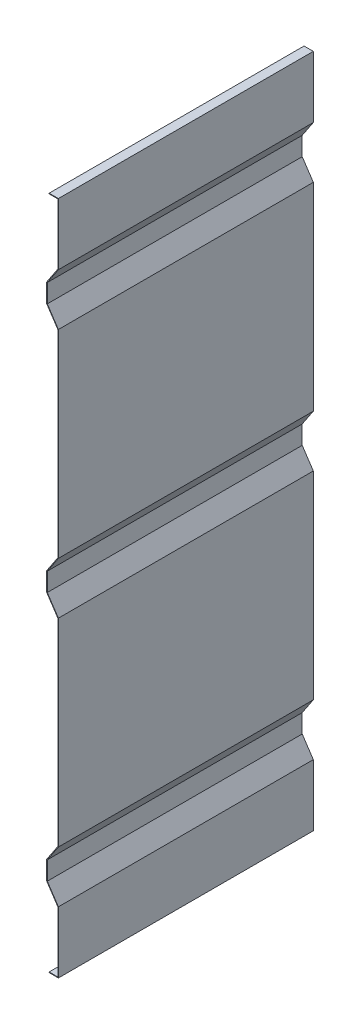
SolidWorks part; units mm, degrees
ref_plane "Front Plane" through (0, 0, 0) normal (0, 0, 1) x (1, 0, 0)
ref_plane "Top Plane" through (0, 0, 0) normal (0, 1, 0) x (1, 0, 0)
ref_plane "Right Plane" through (0, 0, 0) normal (1, 0, 0) x (0, 0, -1)
other "Configuration Table"
sketch "Sketch1" plane through (0, 0, 0) normal (0, 0, 1) x (1, 0, 0)
  line L0 (0, 1095) -> (-30, 1095)
  line L1 (0, 1095) -> (0, 895)
  line L2 (0, 895) -> (-36, 841)
  line L3 (-36, 841) -> (-36, 781)
  line L4 (-36, 781) -> (0, 727)
  line L5 (0, 84) -> (-36, 30)
  line L6 (-36, -30) -> (0, -84)
  line L7 (-36, 30) -> (-36, -30)
  line L8 (-36, 0) -> (85.9436, 0) construction
  line L9 (-36, -781) -> (0, -727)
  line L10 (-36, -841) -> (-36, -781)
  line L11 (0, -895) -> (-36, -841)
  line L12 (0, -1095) -> (-30, -1095)
  line L13 (0, -727) -> (0, -895) construction
  line L14 (0, -895) -> (0, -1095)
  line L15 (0, 895) -> (0, 727) construction
  line L16 (0, 727) -> (0, 84)
  line L17 (0, 0) -> (0, -84) construction
  line L18 (0, -84) -> (0, -727)
  line L19 (0, 84) -> (0, 0) construction
  point P6 (0, 0)
  dimension "D1" = 2190
  dimension "D2" = 36
  dimension "D3" = 54
  dimension "D4" = 54
  dimension "D5" = 60
  dimension "D6" = 200
  dimension "D7" = 30
extrude "Extrude-Thin1" add sketch "Sketch1" along normal mid plane 827 thin thin type one direction wall 2
sketch "Sketch2" plane through (0, 0, 0) normal (1, 0, 0) x (0, 0, -1)
  line L0 (413.5, -84) -> (413.5, -727) construction
  line L1 (-413.5, 1095) -> (413.5, 1095)
  line L2 (-413.5, 1095) -> (-413.5, -645)
  line L3 (-413.5, -645) -> (413.5, -645)
  line L4 (413.5, 1095) -> (413.5, -645)
  dimension "D1" = 1740
extrude "Cut-Extrude1" [suppressed] cut sketch "Sketch2" against normal through all flip side to cut
